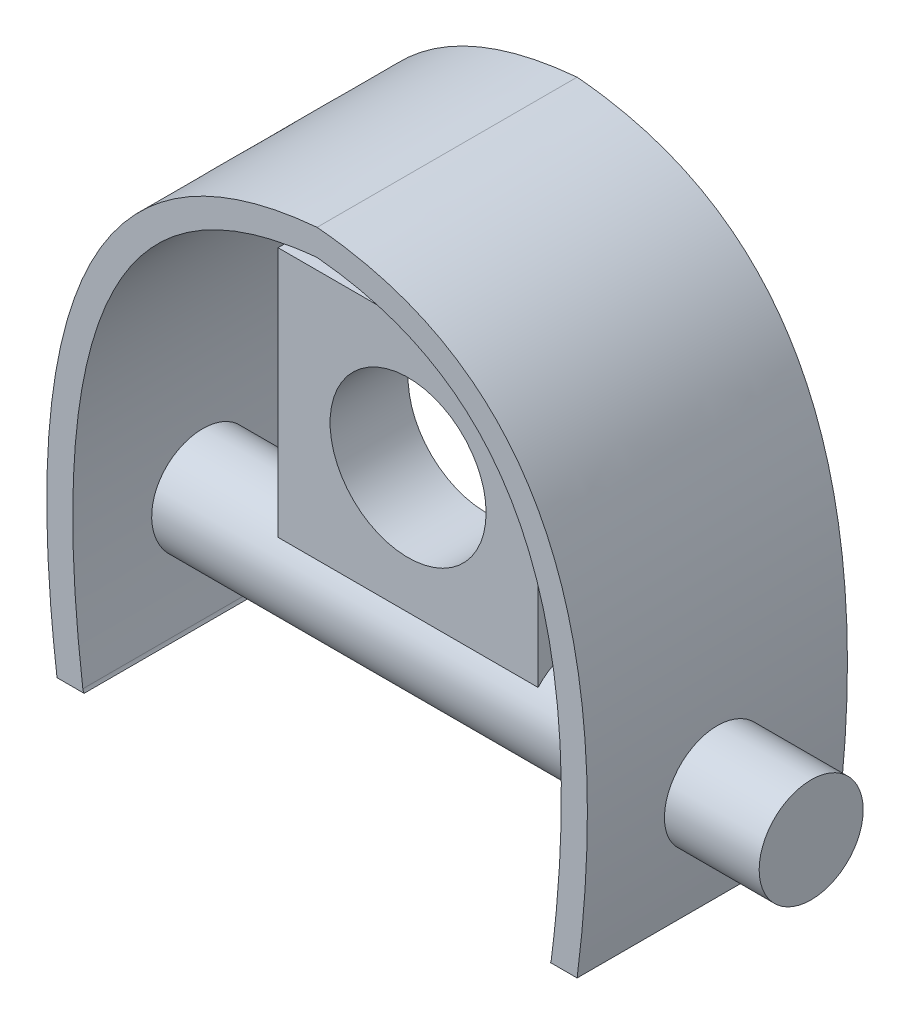
SolidWorks part; units mm, degrees
ref_plane "Front Plane" through (0, 0, 0) normal (0, 0, 1) x (1, 0, 0)
ref_plane "Top Plane" through (0, 0, 0) normal (0, 1, 0) x (1, 0, 0)
ref_plane "Right Plane" through (0, 0, 0) normal (1, 0, 0) x (0, 0, -1)
sketch "Sketch1" plane through (0, 0, 0) normal (0, 0, 1) x (1, 0, 0)
  line L0 (0, 31) -> (0, -35) construction
  line L1 (10, 0) -> (8.9732, 0)
  line L2 (-10, 0) -> (-8.9584, 0)
  arc A0 (9.0081, 0.1269) -> (8.9732, 0) centre (8.543, 0.1864) cw
  arc A1 (-9.0081, 0.1269) -> (-8.9584, 0) centre (-8.7305, 0.1624) ccw
  spline S0 degree 2 poles (0, 20) (12.4195, 18.9088) (10, 0) knots 0 0 0 1 1 1
  spline S1 degree 2 poles (0, 20) (-12.4195, 18.9088) (-10, 0) knots 0 0 0 1 1 1
  spline S2 degree 1 poles (0, 18.9959) (-9.0081, 0.1269) knots 0 0 1 1 construction
  spline S3 degree 1 poles (0, 18.9959) (9.0081, 0.1269) knots 0 0 1 1 construction
  spline S4 degree 3 poles (-9.0081, 0.1269) (-9.0566, 0.5062) (-9.147, 1.2751) (-9.2869, 2.7414) (-9.3919, 4.4921) (-9.4049, 6.4441) (-9.2742, 8.8524) (-8.837, 11.4933) (-7.897, 14.0685) (-6.57, 16.0686) (-4.8629, 17.5479) (-3.0707, 18.3873) (-1.4102, 18.8172) (-0.463, 18.9525) (0, 18.9959) knots 0.003764 0.003764 0.003764 0.003764 0.034896 0.066029 0.128293 0.190558 0.252823 0.377352 0.501882 0.626411 0.750941 0.87547 0.937735 1 1 1 1
  spline S5 degree 3 poles (0, 18.9959) (0.463, 18.9525) (1.4102, 18.8172) (3.0707, 18.3873) (4.8629, 17.5479) (6.57, 16.0686) (7.897, 14.0685) (8.837, 11.4933) (9.2742, 8.8524) (9.4049, 6.4441) (9.3919, 4.4921) (9.2869, 2.7414) (9.147, 1.2751) (9.0566, 0.5062) (9.0081, 0.1269) knots 0.003764 0.003764 0.003764 0.003764 0.066029 0.128293 0.252823 0.377352 0.501882 0.626411 0.750941 0.813206 0.87547 0.937735 0.968868 1 1 1 1
  dimension "D2" = 20
  dimension "D1" = 20
  dimension "D3" = 1
extrude "Boss-Extrude1" add sketch "Sketch1" along normal blind 10
sketch "Sketch3" plane through (0, 0, 0) normal (1, 0, 0) x (0, 0, -1)
  circle A0 centre (-5, 4.1019) radius 2
  dimension "D1" = 4
extrude "Boss-Extrude2" add sketch "Sketch3" along normal blind 14
sketch "Sketch4" plane through (0, 0, 0) normal (-1, 0, 0) x (0, 0, 1)
  circle A0 centre (5, 4.1019) radius 2
  dimension "D1" = 4
extrude "Boss-Extrude3" add sketch "Sketch4" along normal blind 10.5
ref_plane "Plane1" through (0, 0, 5) normal (0, 0, 1) x (1, 0, 0)
sketch "Sketch5" plane through (0, 0, 5) normal (0, 0, 1) x (1, 0, 0)
  line L0 (0, 7.0016) -> (0, -2.9984) construction
  line L2 (-5, 15.07) -> (5, 15.07)
  line L3 (-5, 15.07) -> (-5, 5.07)
  line L4 (-5, 5.07) -> (5, 5.07)
  line L5 (5, 15.07) -> (5, 5.07)
  line L6 (-5, 15.07) -> (5, 5.07) construction
  line L7 (-5, 5.07) -> (5, 15.07) construction
  point P0 (0, 10.07)
  dimension "D1" = 10
  dimension "D2" = 10
extrude "Boss-Extrude4" add sketch "Sketch5" along normal mid plane 3
sketch "Sketch6" plane through (0, 0, 6.5) normal (0, 0, 1) x (1, 0, 0)
  circle A0 centre (0, 10.2474) radius 3
  dimension "D1" = 6
extrude "Cut-Extrude1" cut sketch "Sketch6" against normal blind 17
